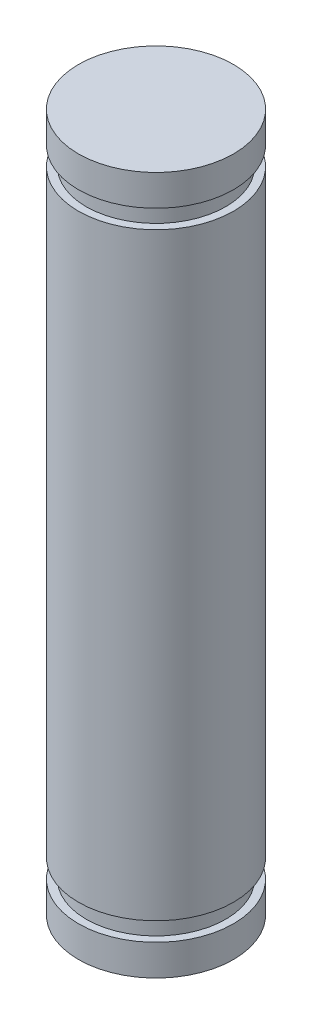
from build123d import *


with BuildPart() as part:
    # 草图1 → 旋转1 (revolve)
    with BuildSketch(Plane(origin=(0, 0, 0), x_dir=(-1, 0, 0), z_dir=(0, 0, -1)), mode=Mode.PRIVATE) as revolve_1_sk:
        Polygon((-5, -22.5), (0, -22.5), (0, 22.5), (-5, 22.5), (-5, 20.5), (-4.5, 20.5), (-4.5, 19.3), (-5, 19.3), (-5, -19.3), (-4.5, -19.3), (-4.5, -20.5), (-5, -20.5), align=None)
    revolve(revolve_1_sk.sketch.rotate(Axis((0, -22.5, 0), (0, 1, 0)), 270), axis=Axis((0, -22.5, 0), (0, 1, 0)))


solid = part.part
